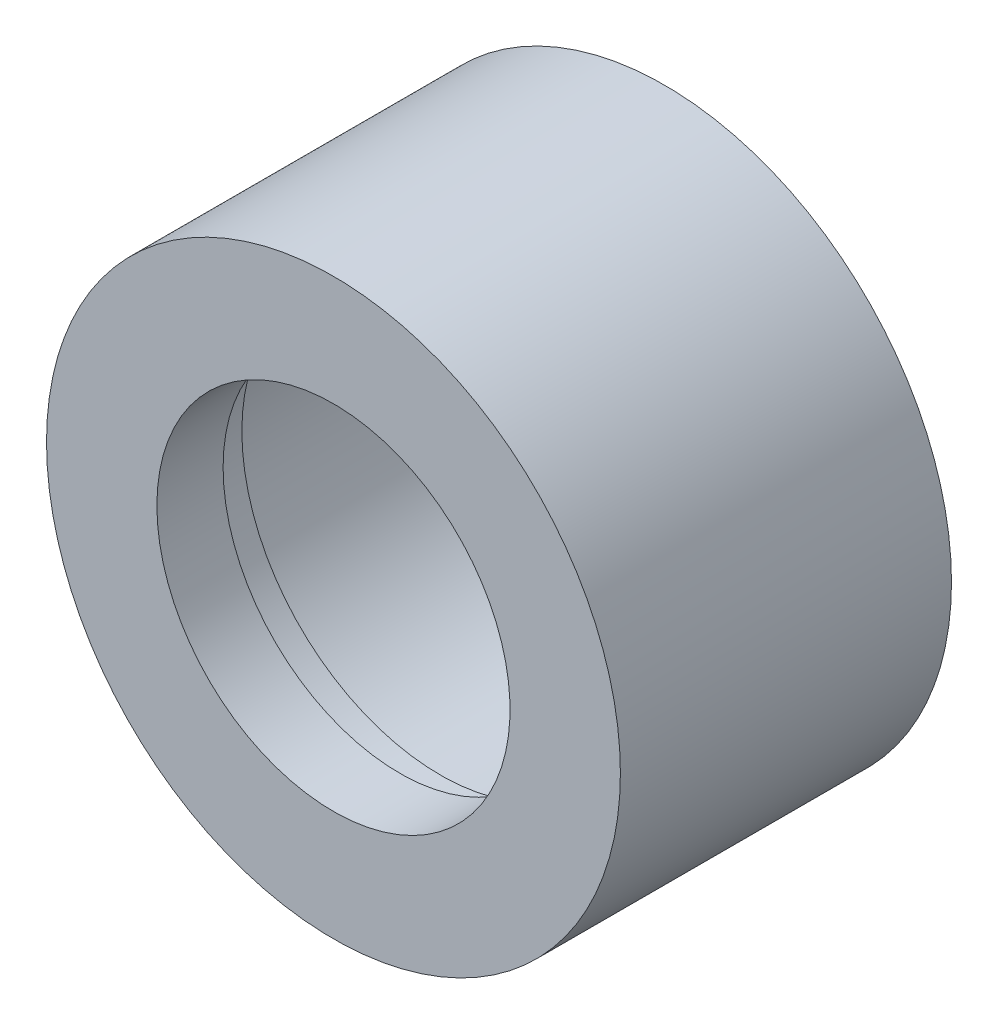
SolidWorks part; units mm, degrees
ref_plane "Front Plane" through (0, 0, 0) normal (0, 0, 1) x (1, 0, 0)
ref_plane "Top Plane" through (0, 0, 0) normal (0, 1, 0) x (1, 0, 0)
ref_plane "Right Plane" through (0, 0, 0) normal (1, 0, 0) x (0, 0, -1)
other "Configuration Table"
ref_plane "Plane1" through (0, 0, 0) normal (0, -1, 0) x (1, 0, 0)
sketch "Sketch1" plane through (0, 0, 0) normal (0, -1, 0) x (1, 0, 0)
  line L0 (9.25, 0) -> (13, 0)
  line L1 (13, 0) -> (13, 15)
  line L2 (13, 15) -> (8, 15)
  line L3 (8, 15) -> (8, 12)
  line L4 (8, 12) -> (9, 12)
  line L5 (9, 12) -> (9, 10.1502)
  line L6 (9, 10.1502) -> (9.25, 10)
  line L7 (9.25, 10) -> (9.25, 0)
  line L8 (0, 15) -> (0, 0) construction
revolve "Revolve1" add sketch "Sketch1" angle 360 about L8
